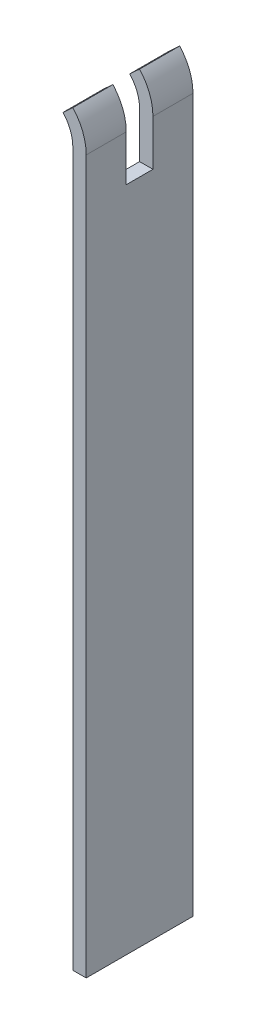
from build123d import *

# Parameters (mm, degrees)
EXTRUDE_1_DEPTH     = 40
CUT_EXTRUDE_1_DEPTH = 40
SKETCH_3_W          = 5
SKETCH_3_H          = 40
EXTRUDE_3_DEPTH     = 6


with BuildPart() as part:
    # 草图1 → 凸台-拉伸1 (new body)
    with BuildSketch(Plane.XY):
        with BuildLine():
            Line((0, 0), (5, 0))
            Line((5, 0), (5, 261))
            ThreePointArc((5, 261), (3.70593121, 267.892024376), (0, 273.845232579))
            Line((0, 273.845232579), (-3.684210526, 270.464908216))
            ThreePointArc((-3.684210526, 270.464908216), (-0.953524372, 266.078333751), (0, 261))
            Line((0, 261), (0, 0))
        make_face()
    extrude(amount=EXTRUDE_1_DEPTH)

    # 草图2 → 切除-拉伸1 (cut)
    with BuildSketch(Plane(origin=(5, 0, 0), x_dir=(0, 0, -1), z_dir=(1, 0, 0))):
        Polygon((-20, 273.845232579), (-25, 273.845232579), (-25, 243.845232579), (-15, 243.845232579), (-15, 273.845232579), align=None)
    extrude(amount=-CUT_EXTRUDE_1_DEPTH, mode=Mode.SUBTRACT)

    # 草图3 → 凸台-拉伸3 (add)
    with BuildSketch(Plane.XZ):
        with Locations((2.5, 20)):
            Rectangle(SKETCH_3_W, SKETCH_3_H)
    extrude(amount=EXTRUDE_3_DEPTH)


solid = part.part
